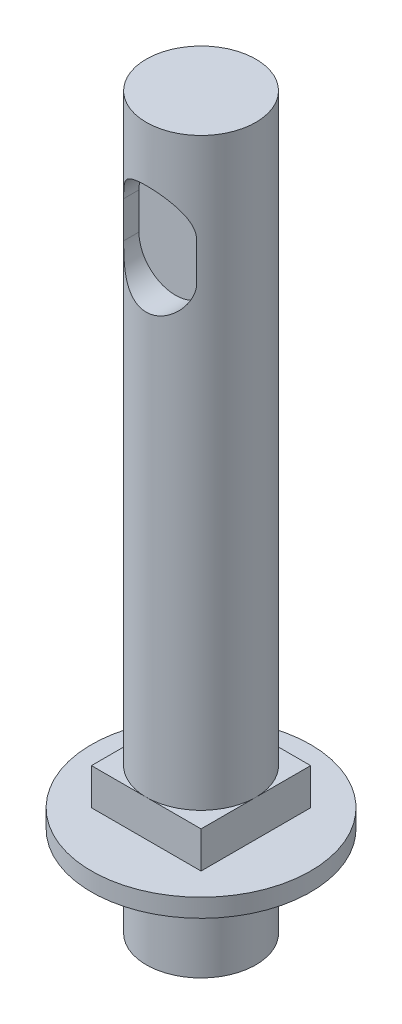
from build123d import *

# Parameters (mm, degrees)
SKETCH2_W           = 6
SKETCH2_H           = 6
BOSS_EXTRUDE1_DEPTH = 2
BOSS_EXTRUDE2_START = 32
SKETCH3_R           = 3
BOSS_EXTRUDE2_DEPTH = 32
CUT_EXTRUDE2_START  = 3
CUT_EXTRUDE2_DEPTH  = 1.6
CUT_EXTRUDE3_START  = -1.4
CUT_EXTRUDE3_DEPTH  = 1.6


with BuildPart() as part:
    # Sketch1 → Revolve1 (revolve)
    with BuildSketch(Plane.XY, mode=Mode.PRIVATE) as revolve1_sk:
        Polygon((0, 0), (3, 0), (3, 4.95), (6, 4.95), (6, 5.95), (0, 5.95), align=None)
    revolve(revolve1_sk.sketch.rotate(Axis((0, -2.859551482, 0), (0, 1, 0)), 90), axis=Axis((0, -2.859551482, 0), (0, 1, 0)))

    # Sketch2 → Boss-Extrude1 (add)
    with BuildSketch(Plane(origin=(0, 5.95, 0), x_dir=(1, 0, 0), z_dir=(0, 1, 0))):
        Rectangle(SKETCH2_W, SKETCH2_H)
    extrude(amount=BOSS_EXTRUDE1_DEPTH)

    # Sketch3 → Boss-Extrude2 (add)
    with BuildSketch(Plane(origin=(0, 7.95, 0), x_dir=(1, 0, 0), z_dir=(0, 1, 0)).offset(BOSS_EXTRUDE2_START)):
        with Locations(Location((0, 0, 0), (0, 0, 90))):
            Circle(SKETCH3_R)
    extrude(amount=-BOSS_EXTRUDE2_DEPTH)

    # Sketch 4_2 → Cut-Extrude2 (cut)
    with BuildSketch(Plane.XY.offset(CUT_EXTRUDE2_START)):
        with BuildLine():
            Line((-2, 32.95), (-2, 34.95))
            ThreePointArc((-2, 34.95), (0, 36.95), (2, 34.95))
            Line((2, 34.95), (2, 32.95))
            ThreePointArc((2, 32.95), (0, 30.95), (-2, 32.95))
        make_face()
    extrude(amount=-CUT_EXTRUDE2_DEPTH, mode=Mode.SUBTRACT)

    # Sketch 4_2 2 → Cut-Extrude3 (cut)
    with BuildSketch(Plane.XY.offset(CUT_EXTRUDE3_START)):
        with BuildLine():
            Line((-2, 32.95), (-2, 34.95))
            ThreePointArc((-2, 34.95), (0, 36.95), (2, 34.95))
            Line((2, 34.95), (2, 32.95))
            ThreePointArc((2, 32.95), (0, 30.95), (-2, 32.95))
        make_face()
    extrude(amount=-CUT_EXTRUDE3_DEPTH, mode=Mode.SUBTRACT)


solid = part.part
